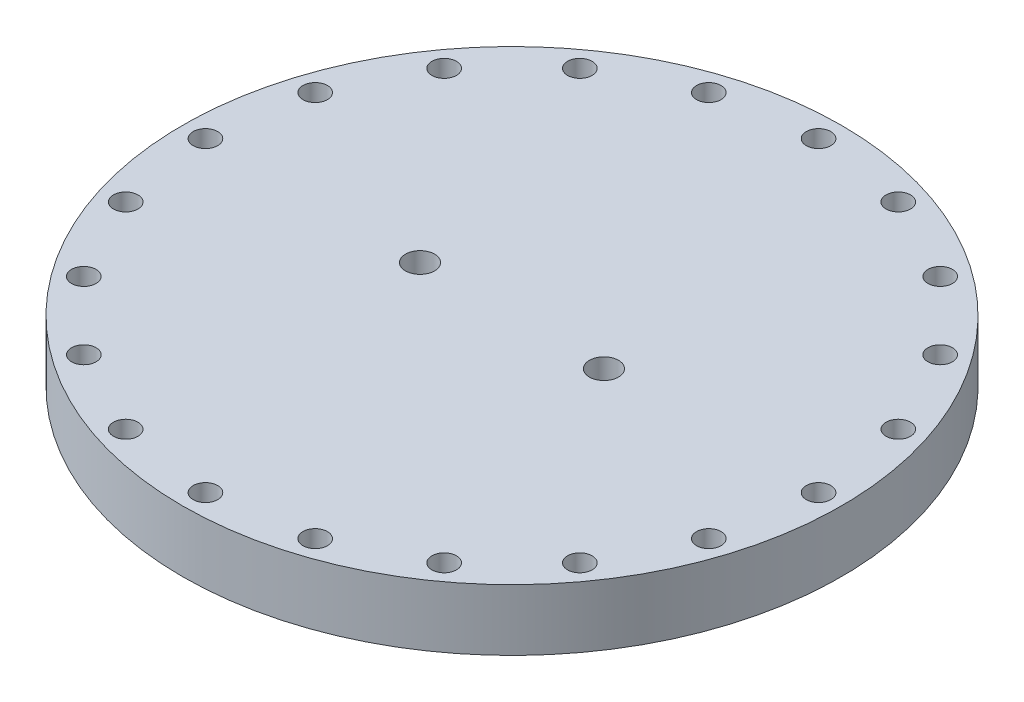
SolidWorks part; units mm, degrees
material "Q235B"
ref_plane "Front Plane" through (0, 0, 0) normal (0, 0, 1) x (1, 0, 0)
ref_plane "Top Plane" through (0, 0, 0) normal (0, 1, 0) x (1, 0, 0)
ref_plane "Right Plane" through (0, 0, 0) normal (1, 0, 0) x (0, 0, -1)
sketch "Sketch1" plane through (0, 0, 0) normal (0, 1, 0) x (1, 0, 0)
  line L1 (215, -400) -> (-215, -400)
  line L2 (215, -400) -> (215, 400)
  line L3 (215, 400) -> (-215, 400)
  line L4 (-215, -400) -> (-215, 400)
  line L5 (215, -400) -> (-215, 400) construction
  line L6 (215, 400) -> (-215, -400) construction
  circle A0 centre (0, 0) radius 215
  circle A1 centre (0, 0) radius 160
  dimension "D1" = 430
  dimension "D4" = 320
  dimension "D2" = 800
  dimension "D3" = 430
extrude "Boss-Extrude1" add sketch "Sketch1" along normal blind 40 contours L2 A0 L4 A1 | A1
hole_wizard "Ø16.0 (16) Diameter Hole1" positions "Sketch3" profile "Sketch4" hole size "Ø16.0" standard "GB" end condition up to next
sketch "Sketch3" plane through (0, 40, 0) normal (0, 1, 0) x (1, 0, 0)
  circle A0 centre (0, 0) radius 200 construction
  point P0 (200, 0)
  point P14 (190.2113, -61.8034)
  point P15 (161.8034, -117.5571)
  point P16 (117.5571, -161.8034)
  point P17 (61.8034, -190.2113)
  point P18 (0, -200)
  point P19 (-61.8034, -190.2113)
  point P20 (-117.5571, -161.8034)
  point P21 (-161.8034, -117.5571)
  point P22 (-190.2113, -61.8034)
  point P23 (-200, 0)
  point P24 (-190.2113, 61.8034)
  point P25 (-161.8034, 117.5571)
  point P26 (-117.5571, 161.8034)
  point P27 (-61.8034, 190.2113)
  point P28 (0, 200)
  point P29 (61.8034, 190.2113)
  point P30 (117.5571, 161.8034)
  point P31 (161.8034, 117.5571)
  point P32 (190.2113, 61.8034)
  dimension "D1" = 400
  dimension "D2" = 20
sketch "Sketch4" plane through (200, 40, 0) normal (1, 0, 0) x (0, 0, 1)
  line L0 (0, 0) -> (0, 40)
  line L1 (0, 40) -> (8, 40)
  line L2 (8, 40) -> (8, 0)
  line L5 (8, 0) -> (0, 0)
  line L11 (0, -6.35) -> (0, 107.95) construction
  dimension "通孔孔直径" = 16
  dimension "通孔孔深度" = 40
hole_wizard "G1/2 Tapped Hole1" positions "Sketch5" profile "Sketch6" tap size "G1/2" standard "GB" end condition up to next
sketch "Sketch5" plane through (0, 40, 0) normal (0, 1, 0) x (1, 0, 0)
  line L0 (0, 50.1035) -> (0, 0) construction
  line L1 (0, 0) -> (-60, 0) construction
  point P0 (-60, 0)
  point P8 (60, 0)
  dimension "D1" = 120
sketch "Sketch6" plane through (-60, 40, 0) normal (1, 0, 0) x (0, 0, 1)
  line L0 (0, 0) -> (0, 40)
  line L1 (0, 40) -> (9.5, 40)
  line L2 (9.5, 40) -> (9.5, 0)
  line L5 (9.5, 0) -> (0, 0)
  line L11 (0, -6.35) -> (0, 107.95) construction
  dimension "通孔螺纹孔钻头直径" = 19
  dimension "通孔螺纹孔钻头深度" = 40
cosmetic thread "CosmeticThread1"
cosmetic thread "CosmeticThread2"
